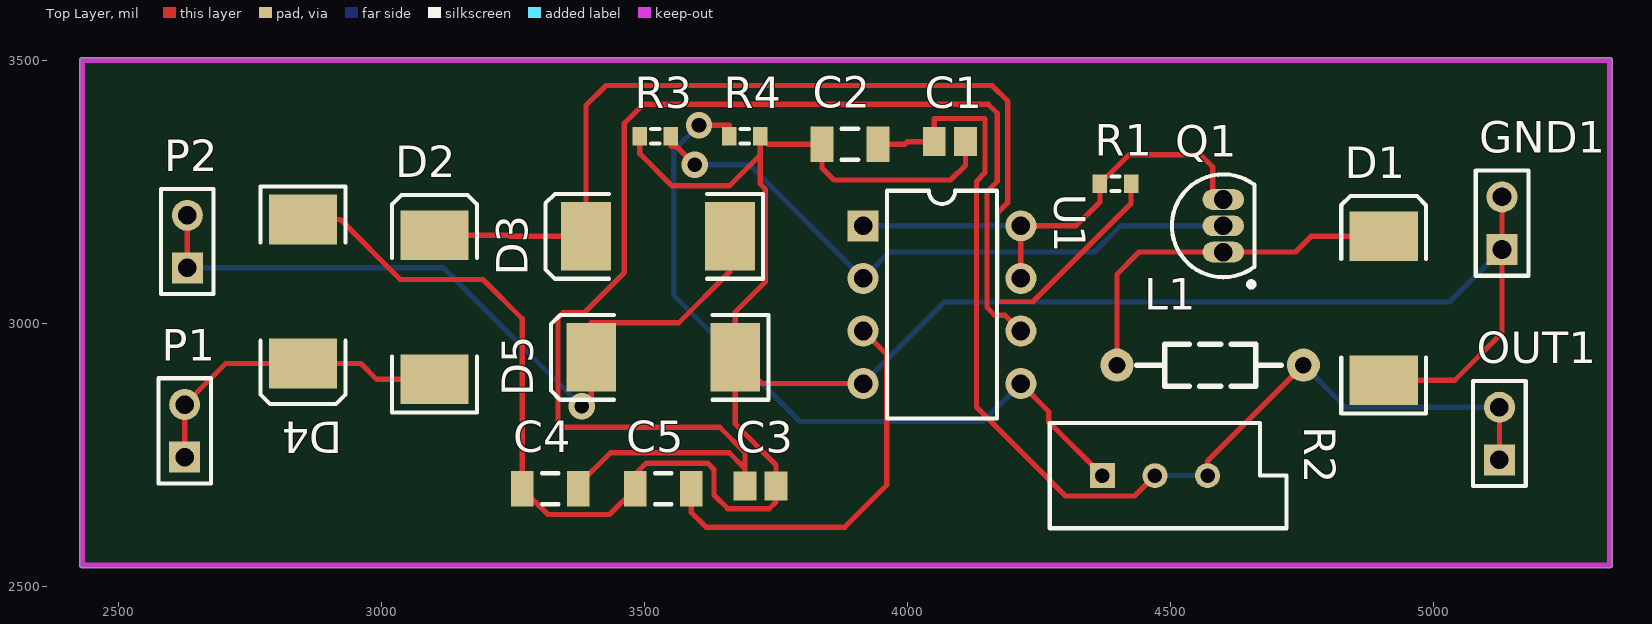
[diagram p0: Top Layer view]
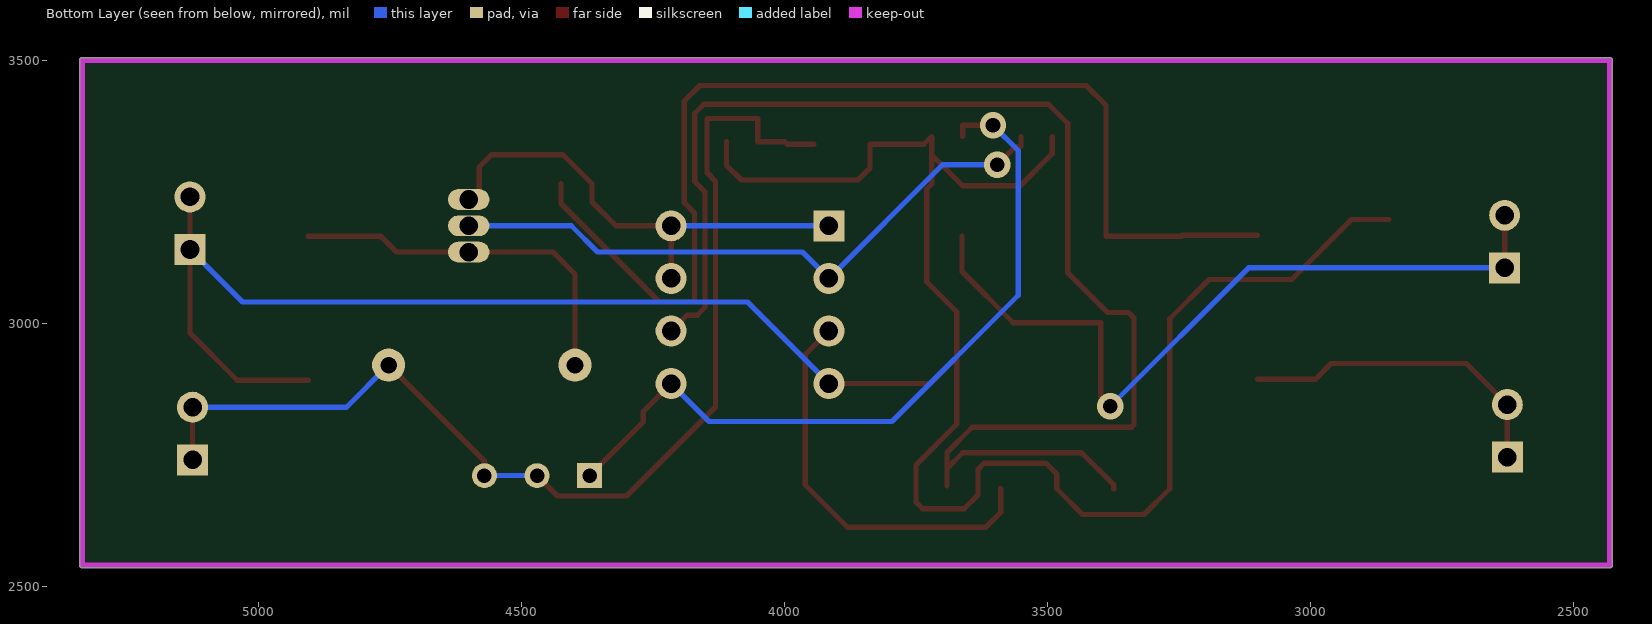
[diagram p1: Bottom Layer view, seen from below]
# Altium PCB MISC89345.PcbDoc
Units mil, origin at the board's own origin, x right, y up, seen from the top; angles counter-clockwise.
Board outline 2915.03 x 970.03 mil, 2 copper layers (Top Layer, Bottom Layer); 21 components, 11 nets, 50 pads, 3 vias.

## Layer stack, top to bottom (the 12.6 mil dielectric is the usual default, probably not edited)
Top Solder: solder mask 0.4, Solder Resist, Dk 3.5
Top Layer: signal copper 1.4
Dielectric 1: dielectric 12.6, FR-4, Dk 4.8
Bottom Layer: signal copper 1.4
Bottom Solder: solder mask 0.4, Solder Resist, Dk 3.5

## Board outline
2430,2534.99 cw(c2430,2540) 2424.99,2540 2424.99,3500 cw(c2430,3500) 2430,3505.01 5335,3505.01 cw(c5335,3500) 5340.02,3500 5340.02,2540 cw(c5335,2540) 5335,2534.99

## Design rules (kind name [scope] priority, off if disabled: settings)
Clearance [All] p1: gap=10
PolygonConnect [All] p1: connectstyle=Relief reliefconductorwidth=10 reliefentries=4 polygonreliefangle="90 Angle" airgapwidth=10
RoutingVias [All] p1: holewidth=28 width=50 viastyle="Through Hole" minholewidth=28 minwidth=50 maxholewidth=28 maxwidth=50
SolderMaskExpansion [All] p1: expansion=4
Width [All] p1: maxlimit=10 minlimit=10 preferedwidth=10
30 further rules are at their usual default settings.

## Components (designator, comment, footprint, x,y, rotation, side; value= is the part's Value field where it differs from the comment)
C1 "1000UF" C0805 4080,3345 r0 top
C2 "104" C1206 3890,3340 r0 top
C3 "470U" C0805 3720,2690 r0 top
C4 "104" C1206 3320,2685 r0 top
C5 "180U" C1206 3535,2685 r0 top
D1 "Diode" SMC 4905,3028.19 r90 top
D2 "Diode" SMC 3100,3030 r90 top
D3 "Diode" SMC 3525,3165 r180 top
D4 "Diode" SMC 2850,3060 r270 top
D5 "Diode" SMC 3535,2935 r180 top
GND1 "Header 2" HDR1X2 5130,3140 r90 top
L1 "470UH" AL0204 4575,2920 r0 top
OUT1 "Header 2" HDR1X2 5125,2740 r90 top
P1 "Header 2" HDR1X2 2625,2745 r90 top
P2 "Header 2" HDR1X2 2630,3105 r90 top
Q1 "2N3904" TO-92A 4600,3185 r0 top
R1 "0.1" J1-0603 4395,3265 r0 top
R2 "RPot" VR5 4470,2710 r0 top
R3 "2K" J1-0603 3520,3355 r0 top
R4 "3.3K" J1-0603 3690,3355 r0 top
U1 "MC34063" 693-02 4065,3035 r270 top

## Footprints (in the part's own frame and the unit in brackets; to place one, negate y for a bottom-side part, rotate by r counter-clockwise, add the part's x,y. Pads: shape width x height; smd on the part's side, far side on the other; paste and mask are expansions set on the pad)
693-02 [mm] "DIP; 8 Leads; Row Spacing 7.62 mm; Pitch 2.54 mm"
  rect 1.5x1.5 hole 0.9: 1(-3.81,-3.81)
  round 1.5 hole 0.9: 2(-1.27,-3.81) 3(1.27,-3.81) 4(3.81,-3.81) 5(3.81,3.81) 6(1.27,3.81) 7(-1.27,3.81) 8(-3.81,3.81)
  silkscreen extent -5.5,-2.65 5.5,2.65
AL0204 [mm] "9*2*4mm（脚距，直径，长度）"
  round 1.6 hole 0.8: 1(-4.5,0) 2(4.5,0)
  silkscreen extent -3.56,-1.02 3.43,1.02, body extent -4.75,-1.02 4.75,1.02, height 2.07
C0805 [mm] "Chip Capacitor, Body 2.0x1.3mm, IPC High Density"
  rect 1.1x1.4 smd: 1(-0.75,0) 2(0.75,0)
  body extent -1.1,-0.72 1.1,0.72, height 1.4
C1206 [mm] "Chip Capacitor, Body 3.2x1.6mm, IPC High Density"
  rect 1.1x1.7 smd: 1(-1.35,0) 2(1.35,0)
  silkscreen extent -0.4,-0.75 0.4,0.75, body extent -1.7,-0.9 1.7,0.9, height 1.3
HDR1X2 [mm] "Connector; Header; 2 Position"
  rect 1.5x1.5 hole 0.9: 1(0,0)
  round 1.5 hole 0.9: 2(2.54,0)
  silkscreen extent -1.27,-1.27 3.81,1.27
J1-0603 [mm] "Chip Resistor, Body 1.6x0.8mm, IPC High Density"
  rect 0.7x0.9 smd: 1(-0.75,0) 2(0.75,0)
  silkscreen extent -0.2,-0.35 0.2,0.35, body extent -0.85,-0.48 0.85,0.48, height 0.9
SMC [mm] "DO-214-AB/SMC; 2 C-Bend Leads; Body 7.9 x 5.9 mm, inc. leads (LxW)"
  rect 2.4x3.3 smd: 1(-3.475,0) 2(3.475,0)
  silkscreen extent -5.07,-2.05 5.43,2.06
TO-92A [mm] "TO, Flat Index; 3 In-Line, Axial Leads; Body Dia. 4.5mm; Leads 0.51 x 0.48 mm (max)"
  oval 2x1 hole 0.9: 1(0,-1.27) 2(0,0) 3(0,1.27)
  silkscreen extent -2.48,-2.95 1.5,2.48, body extent -2.48,-2.5 1.5,2.5, height 6.86
VR5 [mm] "Thru-Hole; 3 Leads"
  rect 1.2x1.2 hole 0.7: 1(-2.54,0)
  round 1.2 hole 0.7: 2(0,0) 3(2.54,0)
  silkscreen extent -5.08,-2.54 6.35,2.54

## Part data
C1 C3: library part "Cap Pol3", "Polarized Capacitor (Surface Mount)"
C2 C4 C5: library part "Cap Semi", "Capacitor (Semiconductor SIM Model)"
D1 D2 D3 D4 D5: "Default Diode"
GND1 OUT1 P1 P2: "Header, 2-Pin"
L1: library part INDUCTOR, "INDUCTOR"
Q1: "NPN General Purpose Amplifier"
R1 R3 R4: library part Res2, "Resistor"
R2: "Potentiometer"
U1: library part MC34063U, "DC-to-DC Converter Control Circuit"

## Via types
v1: diameter 50, hole 28, Top Layer to Bottom Layer, 3 vias

## Nets (pads, with @x,y where several pads share a name; then routed paths per layer and width w, separated by ;. In a path a pad name is that pad's centre, name@x,y a point inside that pad or via, vN(x,y) a via of type N, cw(c..) or ccw(c..) an arc to the next point about the centre after c; other vN are vias at no path point)
NetC1_1: C1.1 C2.2 L1.2 OUT1.1 OUT1.2 R2.2 R2.3 | length 2122.6
  Top Layer w10: C2.2 3994,3340 3999,3345 C1.1 4050.47,3389 4147,3389 4147,3286.06 4130.47,3269.53 4130.47,2840.53 4300,2671 4431,2671 R2.2 ; R2.3 4570,2737.83 L1.2 ; OUT1.1 OUT1.2
  Bottom Layer w10: R2.2 R2.3 ; L1.2 4832.17,2840 OUT1.2
NetC1_2: C1.2 C2.1 C3.2 C4.1 C5.1 D1.1 D4.1 D5.1 GND1.1 GND1.2 R3.1 R4.2 U1.4 | length 5126.8
  Top Layer w10: D4.1 2921,3196.81 3034.81,3083 3192,3083 3266.85,3008.15 C4.1 3315.85,2636 3432.85,2636 C5.1 3481.85,2713 3502.32,2733.47 3620,2733.47 3631.62,2721.85 3631.62,2673.19 3657.81,2647 3736.53,2647 3749.53,2660 C3.2 3749.53,2730.28 3671.81,2808 D5.1 ; R3.1 3490.47,3322 3551.47,3261 3660.55,3261 3719.53,3319.97 ; U1.4 3721.81,2885 D5.1 ; C1.2 4109.53,3300 4081.53,3272 3860,3272 3836.85,3295.15 C2.1 3734.53,3340 R4.2 3719.53,3319.97 ; D1.1 5040,2891.38 5130,2981.38 GND1.1 GND1.2 ; D5.1 3671.81,3021 3729,3078.19 3729,3255 3719.53,3264.47 3719.53,3319.97
  Bottom Layer w10: U1.4 4070,3040 5030,3040 GND1.1
NetC3_1: C3.1 C4.2 U1.6 | length 2643.3
  Top Layer w10: C4.2 3373.15,2692 3434.62,2753.47 3660.53,2753.47 3690.47,2723.53 ; C3.1 3690.47,2723.53 ; U1.6 4185,3015 4165.47,3015 4150.47,3030 4150.47,3249.53 4170,3269.06 4170,3399 4153,3416 3497,3416 3461,3380 3461,3096.04 3384.96,3020 3345,3020 3335,3010 3335,2807.24 3340.24,2802 3642.47,2802 3690.47,2754 3690.47,2723.53
NetC5_2: C5.2 U1.3 | length 773.2
  Top Layer w10: C5.2 3588.15,2640 3616.15,2612 3880,2612 3960,2692 3960,2940 U1.3
NetD1_2: D1.2 L1.1 Q1.1 | length 709.9
  Top Layer w10: L1.1 4397.83,3092.83 4440,3135 Q1.1 4737,3135 4767,3165 D1.2
NetD2_1: D2.1 D4.2 P1.1 P1.2 | length 619.8
  Top Layer w10: P1.1 P1.2 2703.19,2923.19 D4.2 2960,2923.19 2990,2893.19 D2.1
NetD2_2: D2.2 D3.2 R1.2 | length 2126.3
  Top Layer w10: D2.2 3243,3166.81 3244.81,3165 D3.2 3388.19,3414.19 3426,3452 4160,3452 4190,3422 4190,3229 4170.47,3209.47 4170.47,3041 4237,3040 4424.53,3227.53 R1.2
NetD3_1: D3.1 D5.2 P2.1 P2.2 | length 1496.1
  Top Layer w10: P2.1 P2.2 ; v1(3380,2842) 3398.19,2860.19 D5.2 3398.19,3000.57 3564.57,3000.57 3661.81,3097.81 D3.1
  Bottom Layer w10: P2.1 3117,3105 v1(3380,2842)
NetQ1_2: Q1.2 R3.2 U1.2 | length 1214.9
  Top Layer w10: R3.2 3549.53,3335.91 3560.09,3335.91 v1(3595,3301)
  Bottom Layer w10: v1(3595,3301) 3699,3301 U1.2 3965,3135 4355,3135 4405,3185 Q1.2
NetQ1_3: Q1.3 R1.1 U1.1 U1.7 U1.8 | length 932.4
  Top Layer w10: U1.7 U1.8 4320,3185 4365.47,3230.47 R1.1 4420.47,3320 4556.47,3320 4580,3296.47 4580,3235 Q1.3
  Bottom Layer w10: U1.1 U1.8
NetR2_1: R2.1 R4.1 U1.5 | length 1449.8
  Top Layer w10: v1(3603,3376) 3660.47,3376 R4.1 ; U1.5 4268,2832 4268,2812 R2.1
  Bottom Layer w10: v1(3603,3376) 3555,3328 3555,3053 3795,2813 4143,2813 U1.5

## Keep-outs
Keep-Out Layer:
  lines w10: 2430,2540 2430,3500 5335,3500 5335,2540 2430,2540